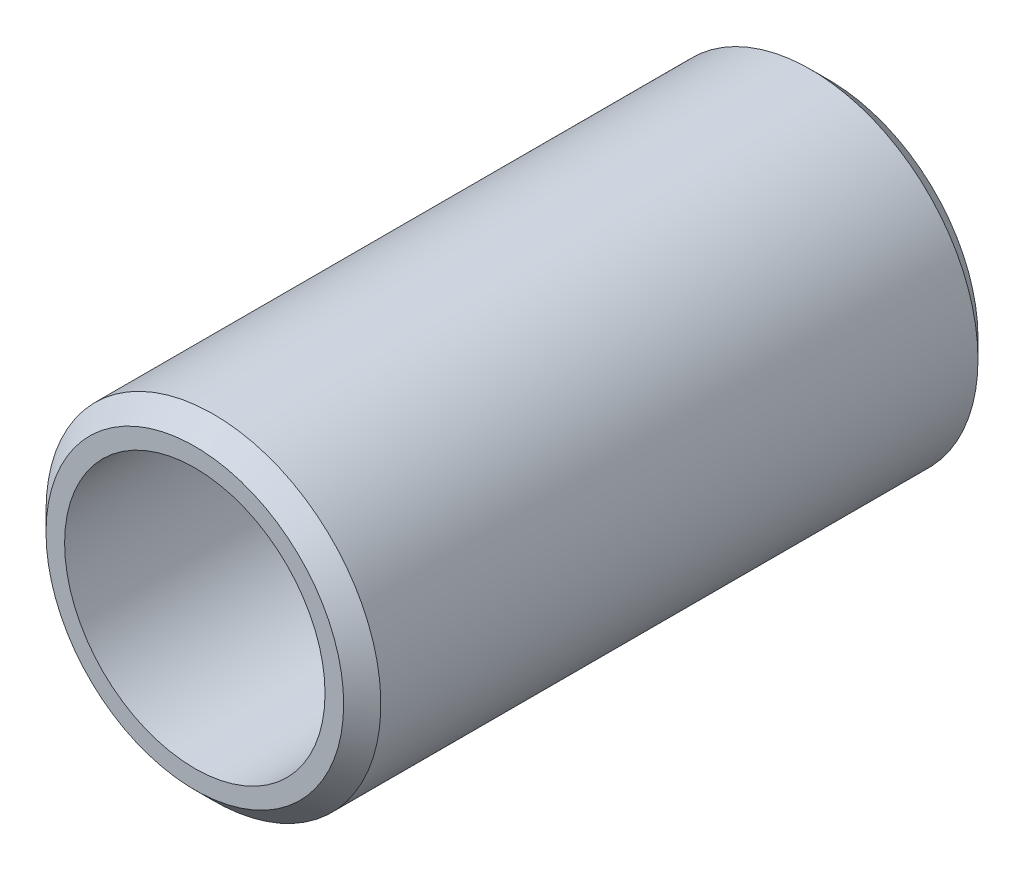
from build123d import *

# Parameters (mm, degrees)
SKETCH2_R           = 90
SKETCH2_R_2         = 70
BOSS_EXTRUDE1_DEPTH = 341
CHAMFER1_SIZE       = 10


with BuildPart() as part:
    # Sketch2 → Boss-Extrude1 (new body)
    with BuildSketch(Plane.XY):
        with Locations(Location((0, 0, 0), (0, 0, 180))):
            Circle(SKETCH2_R)
        with Locations(Location((0, 0, 0), (0, 0, 180))):
            Circle(SKETCH2_R_2, mode=Mode.SUBTRACT)
    extrude(amount=BOSS_EXTRUDE1_DEPTH)

    # Chamfer1
    chamfer1_edges = [part.edges().sort_by_distance(p)[0] for p in [
        (90, 0, 0),
        (90, 0, 341),
    ]]
    chamfer(chamfer1_edges, length=CHAMFER1_SIZE)


solid = part.part
